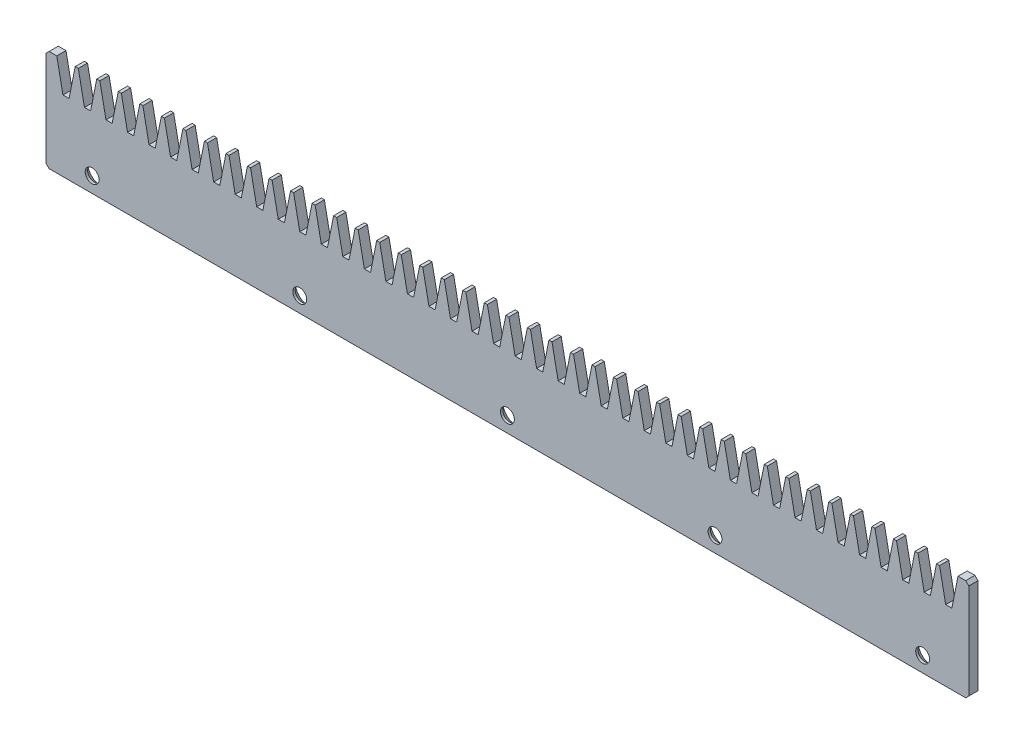
from build123d import *

# Parameters (mm, degrees)
SKETCH_2_W                   = 300
SKETCH_2_H                   = 33
EXTRUDE_1_DEPTH              = 3
CUT_EXTRUDE_1_DEPTH          = 15
CHAMFER_1_SIZE               = 1
HOLE_WIZARD_M4_1_D           = 4.5
HOLE_WIZARD_M4_1_DEPTH       = 11.5
HOLE_WIZARD_M4_1_CSINK_D     = 8.96
HOLE_WIZARD_M4_1_CSINK_ANGLE = 90
HOLE_WIZARD_M4_1_TIP         = 1.351936393


with BuildPart() as part:
    # 草图2 → 凸台-拉伸1 (new body)
    with BuildSketch(Plane.XY):
        with Locations((150, 16.5)):
            Rectangle(SKETCH_2_W, SKETCH_2_H)
    extrude(amount=EXTRUDE_1_DEPTH)

    # 草图3 → 切除-拉伸1 (cut)
    with BuildSketch(Plane.XY.offset(3)):
        Polygon((3.5, 33), (9.5, 33), (7.5, 23), (5.5, 23), align=None)
        Polygon((12.5, 23), (10.5, 33), (16.5, 33), (14.5, 23), align=None)
        Polygon((19.5, 23), (17.5, 33), (23.5, 33), (21.5, 23), align=None)
        Polygon((26.5, 23), (24.5, 33), (30.5, 33), (28.5, 23), align=None)
        Polygon((33.5, 23), (31.5, 33), (37.5, 33), (35.5, 23), align=None)
        Polygon((40.5, 23), (38.5, 33), (44.5, 33), (42.5, 23), align=None)
        Polygon((47.5, 23), (45.5, 33), (51.5, 33), (49.5, 23), align=None)
        Polygon((54.5, 23), (52.5, 33), (58.5, 33), (56.5, 23), align=None)
        Polygon((61.5, 23), (59.5, 33), (65.5, 33), (63.5, 23), align=None)
        Polygon((68.5, 23), (66.5, 33), (72.5, 33), (70.5, 23), align=None)
        Polygon((75.5, 23), (73.5, 33), (79.5, 33), (77.5, 23), align=None)
        Polygon((82.5, 23), (80.5, 33), (86.5, 33), (84.5, 23), align=None)
        Polygon((89.5, 23), (87.5, 33), (93.5, 33), (91.5, 23), align=None)
        Polygon((96.5, 23), (94.5, 33), (100.5, 33), (98.5, 23), align=None)
        Polygon((103.5, 23), (101.5, 33), (107.5, 33), (105.5, 23), align=None)
        Polygon((110.5, 23), (108.5, 33), (114.5, 33), (112.5, 23), align=None)
        Polygon((117.5, 23), (115.5, 33), (121.5, 33), (119.5, 23), align=None)
        Polygon((124.5, 23), (122.5, 33), (128.5, 33), (126.5, 23), align=None)
        Polygon((131.5, 23), (129.5, 33), (135.5, 33), (133.5, 23), align=None)
        Polygon((138.5, 23), (136.5, 33), (142.5, 33), (140.5, 23), align=None)
        Polygon((145.5, 23), (143.5, 33), (149.5, 33), (147.5, 23), align=None)
        Polygon((152.5, 23), (150.5, 33), (156.5, 33), (154.5, 23), align=None)
        Polygon((159.5, 23), (157.5, 33), (163.5, 33), (161.5, 23), align=None)
        Polygon((166.5, 23), (164.5, 33), (170.5, 33), (168.5, 23), align=None)
        Polygon((173.5, 23), (171.5, 33), (177.5, 33), (175.5, 23), align=None)
        Polygon((180.5, 23), (178.5, 33), (184.5, 33), (182.5, 23), align=None)
        Polygon((187.5, 23), (185.5, 33), (191.5, 33), (189.5, 23), align=None)
        Polygon((194.5, 23), (192.5, 33), (198.5, 33), (196.5, 23), align=None)
        Polygon((201.5, 23), (199.5, 33), (205.5, 33), (203.5, 23), align=None)
        Polygon((208.5, 23), (206.5, 33), (212.5, 33), (210.5, 23), align=None)
        Polygon((215.5, 23), (213.5, 33), (219.5, 33), (217.5, 23), align=None)
        Polygon((222.5, 23), (220.5, 33), (226.5, 33), (224.5, 23), align=None)
        Polygon((229.5, 23), (227.5, 33), (233.5, 33), (231.5, 23), align=None)
        Polygon((236.5, 23), (234.5, 33), (240.5, 33), (238.5, 23), align=None)
        Polygon((243.5, 23), (241.5, 33), (247.5, 33), (245.5, 23), align=None)
        Polygon((250.5, 23), (248.5, 33), (254.5, 33), (252.5, 23), align=None)
        Polygon((257.5, 23), (255.5, 33), (261.5, 33), (259.5, 23), align=None)
        Polygon((264.5, 23), (262.5, 33), (268.5, 33), (266.5, 23), align=None)
        Polygon((271.5, 23), (269.5, 33), (275.5, 33), (273.5, 23), align=None)
        Polygon((278.5, 23), (276.5, 33), (282.5, 33), (280.5, 23), align=None)
        Polygon((285.5, 23), (283.5, 33), (289.5, 33), (287.5, 23), align=None)
        Polygon((292.5, 23), (290.5, 33), (296.5, 33), (294.5, 23), align=None)
    extrude(amount=-CUT_EXTRUDE_1_DEPTH, mode=Mode.SUBTRACT)

    # 倒角1
    chamfer_1_edges = [part.edges().sort_by_distance(p)[0] for p in [
        (0, 33, 1.5),
        (300, 33, 1.5),
        (300, 0, 1.5),
        (0, 0, 1.5),
    ]]
    chamfer(chamfer_1_edges, length=CHAMFER_1_SIZE)

    # M4 六角凹锥坑螺钉的锥形沉头孔1
    with Locations(Plane(origin=(0, 0, 0), x_dir=(-1, 0, 0), z_dir=(0, 0, -1))):
        with Locations((-285, 5), (-217.5, 5), (-150, 5), (-82.5, 5), (-15, 5)):
            CounterSinkHole(HOLE_WIZARD_M4_1_D / 2, HOLE_WIZARD_M4_1_CSINK_D / 2, depth=HOLE_WIZARD_M4_1_DEPTH, counter_sink_angle=HOLE_WIZARD_M4_1_CSINK_ANGLE)
            with Locations((0, 0, -(HOLE_WIZARD_M4_1_DEPTH + HOLE_WIZARD_M4_1_TIP / 2))):  # 118° drill point
                Cone(0, HOLE_WIZARD_M4_1_D / 2, HOLE_WIZARD_M4_1_TIP, mode=Mode.SUBTRACT)


solid = part.part
